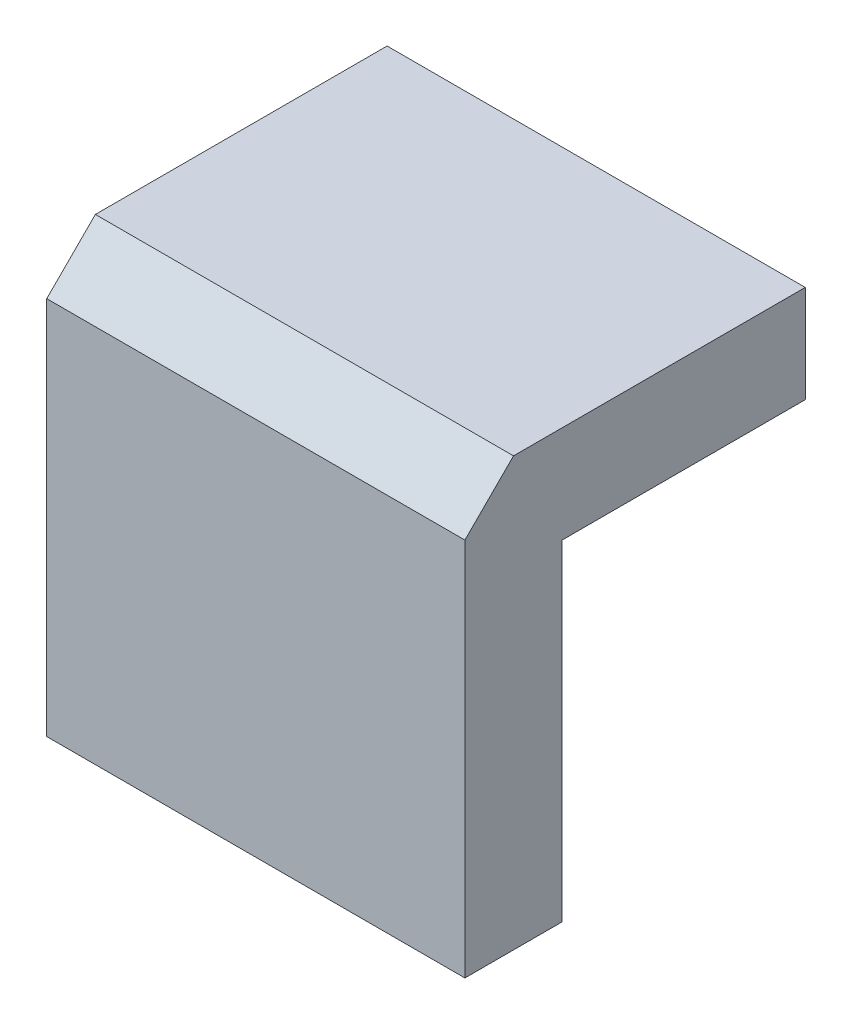
from build123d import *

# Parameters (mm, degrees)
SKETCH_1_W             = 43
SKETCH_1_H             = 44
EXTRUDE_1_DEPTH        = 17.5
SKETCH_2_W             = 50
SKETCH_2_H             = 68
CUT_EXTRUDE_1_DEPTH    = 52.373631369
HOLE_WIZARD_M4_1_D     = 3.3
HOLE_WIZARD_M4_1_DEPTH = 15.5
HOLE_WIZARD_M4_1_TIP   = 0.991420021
CHAMFER_1_SIZE         = 5
HOLE_WIZARD_M4_2_D     = 3.3
HOLE_WIZARD_M4_2_DEPTH = 15.5
HOLE_WIZARD_M4_2_TIP   = 0.991420021


with BuildPart() as part:
    # 草图1 → 凸台-拉伸1 (new, symmetric)
    with BuildSketch(Plane.XY):
        Rectangle(SKETCH_1_W, SKETCH_1_H)
    extrude(amount=EXTRUDE_1_DEPTH, both=True)

    # 草图2 → 切除-拉伸1 (cut, through all)
    with BuildSketch(Plane(origin=(21.5, 0, 0), x_dir=(0, 0, -1), z_dir=(1, 0, 0))):
        with Locations((17.5, -22)):
            Rectangle(SKETCH_2_W, SKETCH_2_H)
    extrude(amount=-CUT_EXTRUDE_1_DEPTH, mode=Mode.SUBTRACT)

    # M4 螺纹孔1
    with Locations(Plane(origin=(0, 0, -17.5), x_dir=(-1, 0, 0), z_dir=(0, 0, -1))):
        with Locations((-15, 17), (15, 17)):
            Hole(HOLE_WIZARD_M4_1_D / 2, depth=HOLE_WIZARD_M4_1_DEPTH)
            with Locations((0, 0, -(HOLE_WIZARD_M4_1_DEPTH + HOLE_WIZARD_M4_1_TIP / 2))):  # 118° drill point
                Cone(0, HOLE_WIZARD_M4_1_D / 2, HOLE_WIZARD_M4_1_TIP, mode=Mode.SUBTRACT)

    # 倒角1
    chamfer_1_edges = [part.edges().sort_by_distance(p)[0] for p in [
        (0, 22, 17.5),
    ]]
    chamfer(chamfer_1_edges, length=CHAMFER_1_SIZE)

    # M4 螺纹孔2
    with Locations(Plane(origin=(0, -22, 0), x_dir=(-1, 0, 0), z_dir=(0, -1, 0))):
        with Locations((10, -12.5), (-10, -12.5)):
            Hole(HOLE_WIZARD_M4_2_D / 2, depth=HOLE_WIZARD_M4_2_DEPTH)
            with Locations((0, 0, -(HOLE_WIZARD_M4_2_DEPTH + HOLE_WIZARD_M4_2_TIP / 2))):  # 118° drill point
                Cone(0, HOLE_WIZARD_M4_2_D / 2, HOLE_WIZARD_M4_2_TIP, mode=Mode.SUBTRACT)


solid = part.part
